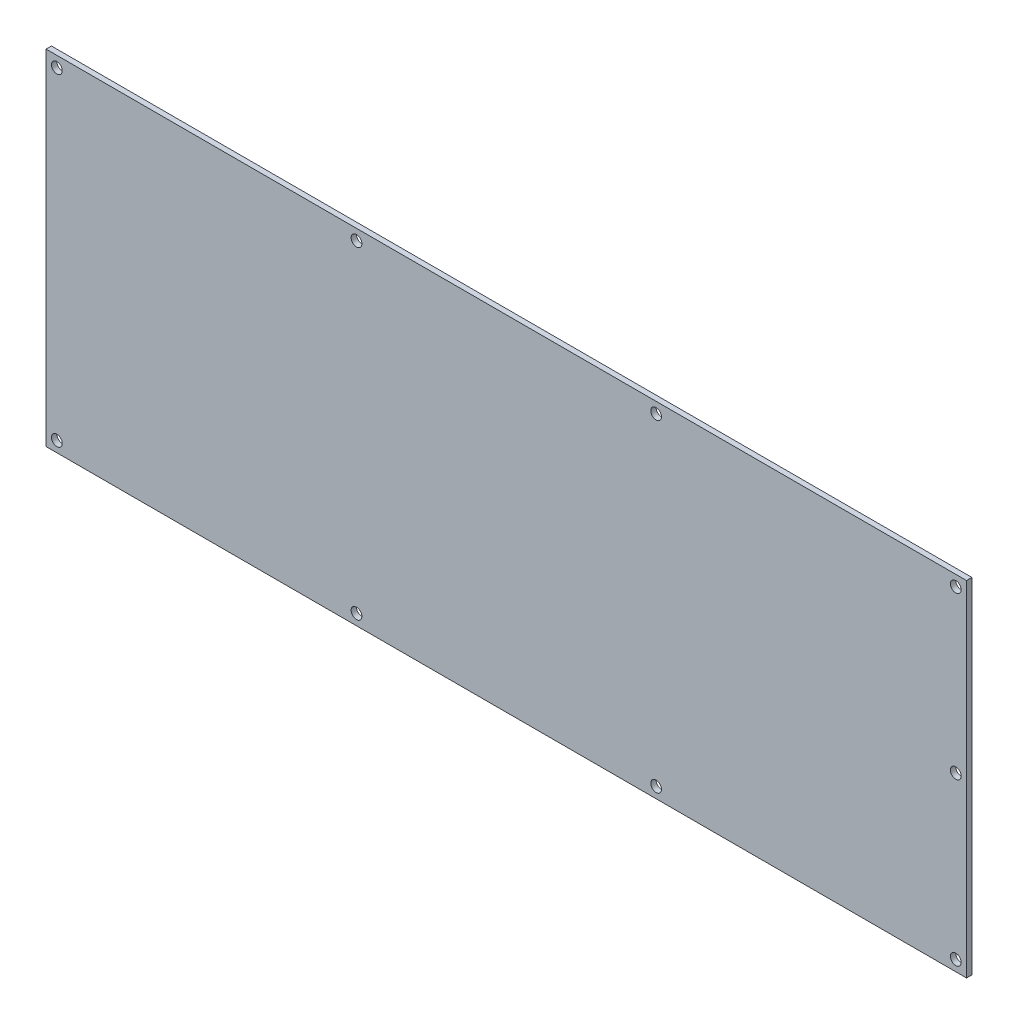
SolidWorks part; units mm, degrees
ref_plane "Front Plane" through (0, 0, 0) normal (0, 0, 1) x (1, 0, 0)
ref_plane "Top Plane" through (0, 0, 0) normal (0, 1, 0) x (1, 0, 0)
ref_plane "Right Plane" through (0, 0, 0) normal (1, 0, 0) x (0, 0, -1)
other "Configuration Table"
sketch "Sketch1" plane through (0, 0, 0) normal (0, 0, 1) x (1, 0, 0)
  line L0 (0, 319.7616) -> (855.0225, 319.7616)
  line L1 (855.0225, 319.7616) -> (855.0225, 0)
  line L2 (855.0225, 0) -> (0, 0)
  line L3 (0, 0) -> (0, 319.7616)
  circle A0 centre (10, 309.7616) radius 5
  circle A1 centre (845.0225, 309.7616) radius 5
  circle A2 centre (10, 10) radius 5
  circle A3 centre (845.0225, 10) radius 5
  circle A4 centre (288.3408, 309.7616) radius 5
  circle A5 centre (288.3408, 10) radius 5
  circle A6 centre (566.6816, 309.7616) radius 5
  circle A7 centre (566.6816, 10) radius 5
  circle A8 centre (845.0225, 159.8808) radius 5
  dimension "D1" = 10
  dimension "D2" = 10
  dimension "D3" = 288.3408
  dimension "D4" = 566.6816
  dimension "D5" = 845.0225
  dimension "D6" = 855.0225
  dimension "D7" = 10
  dimension "D8" = 159.8808
  dimension "D9" = 309.7616
  dimension "D10" = 319.7616
extrude "Boss-Extrude1" add sketch "Sketch1" along normal blind 5
